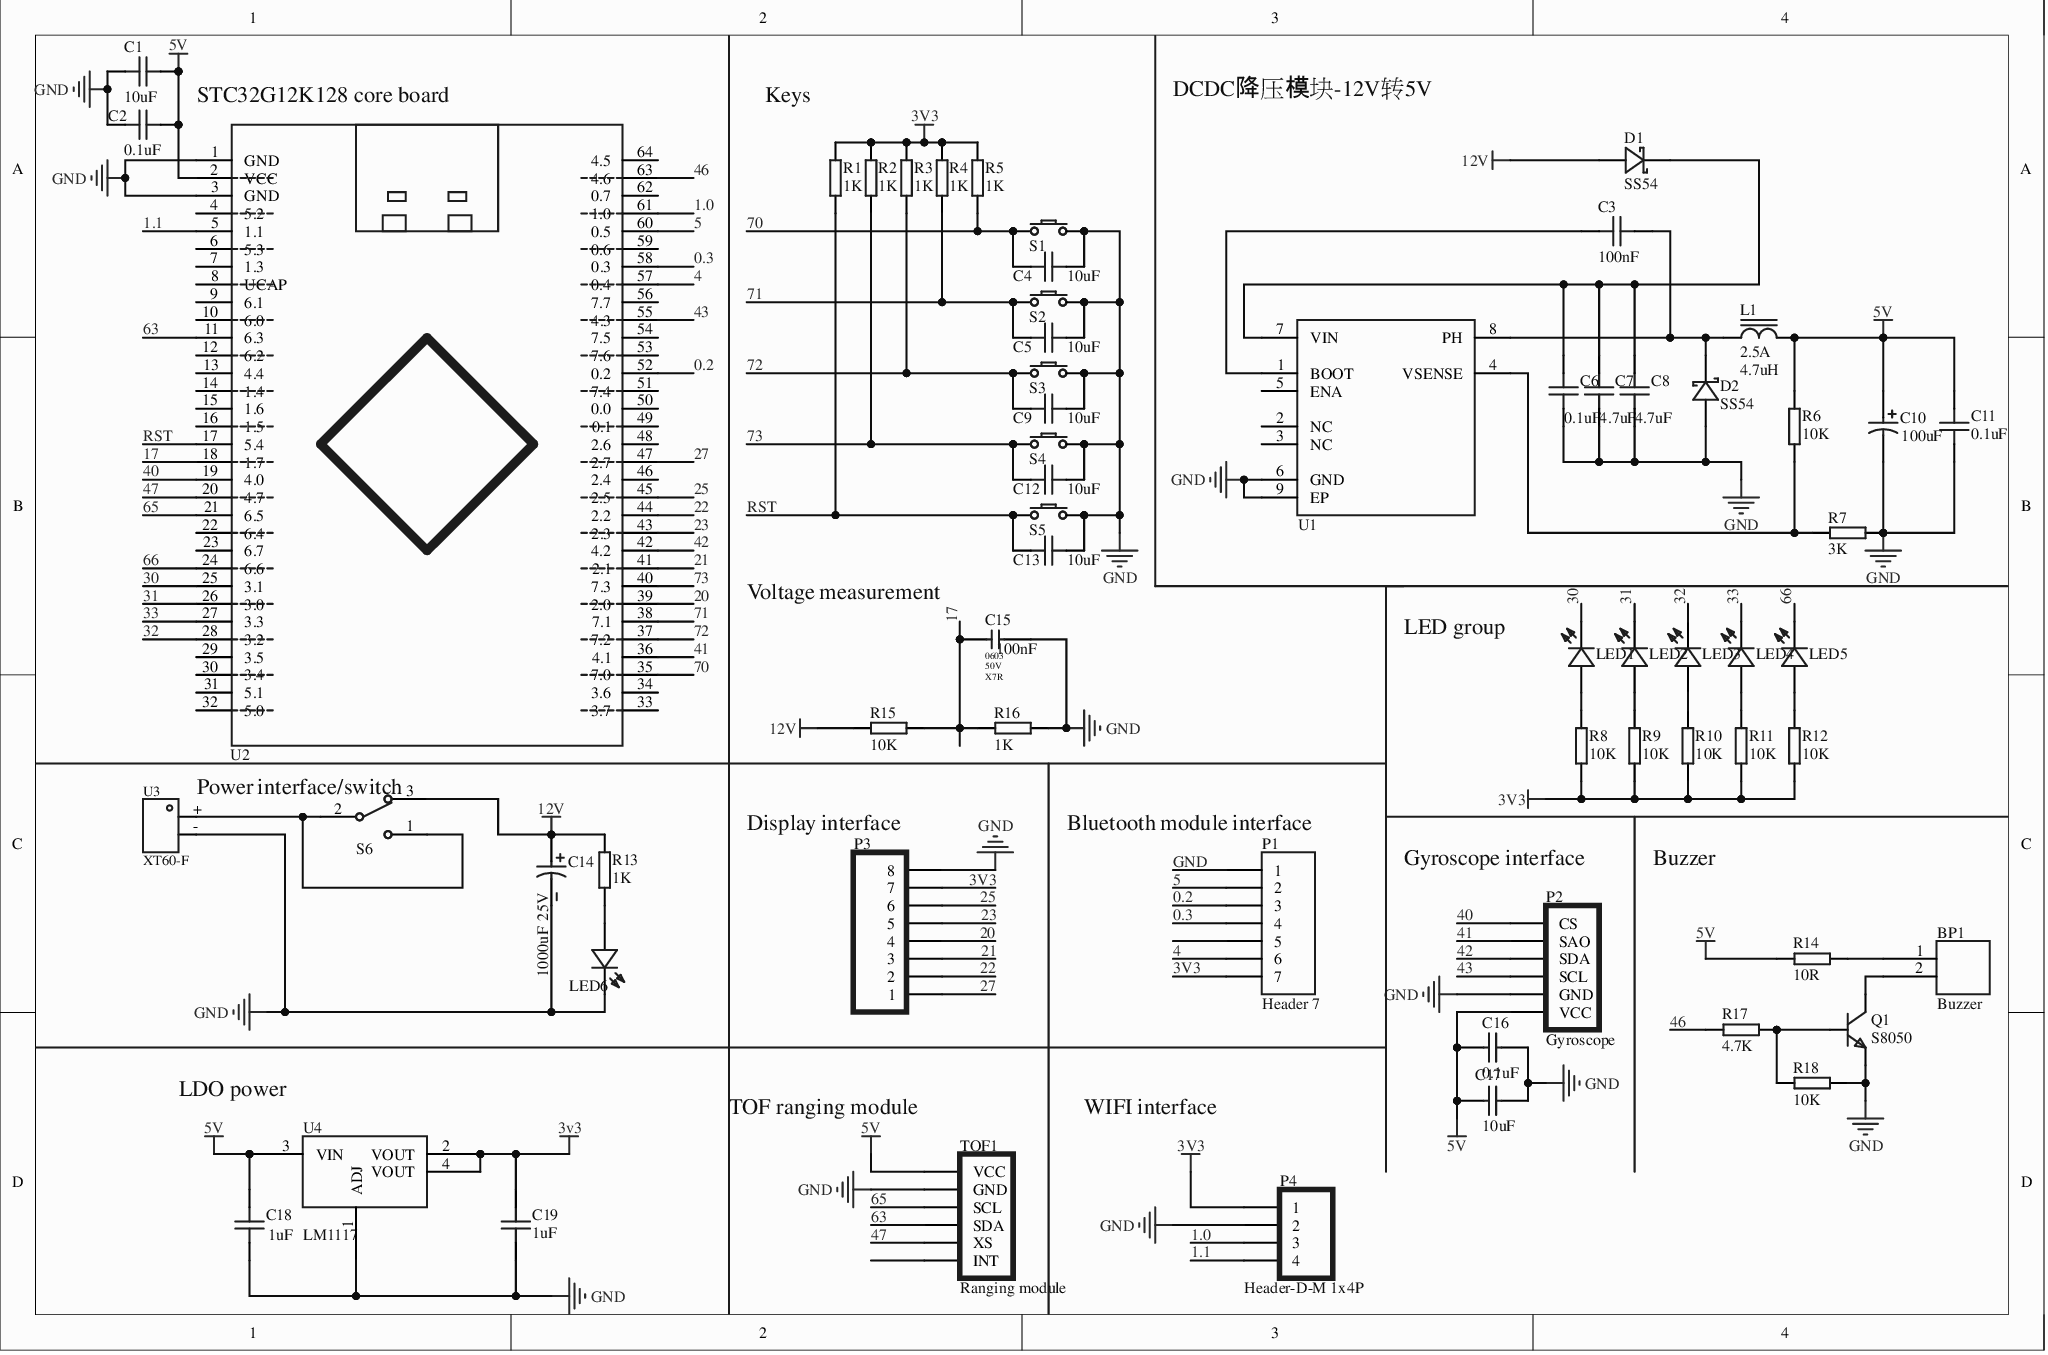
[diagram p0: MISC75116-2.schdoc]
# Altium project MISC75116-3.PrjPcb
1 sheet, 63 parts. Net scope: global (net labels, ports and power ports of the same name join across sheets).
Board file: MISC75116.pcbdoc

## Sheet MISC75116-2.schdoc
size 292 x 193 mm; Name: MISC75116

### Parts
BP1  Buzzer  [5*10fengmiqi]
C1  10uF  [CAPC1608[0603]S-N]
C2  0.1uF  [CAPC1608[0603]S-N]
C3  100nF  [CAPC1608[0603]S-N]
C4  10uF  [CAPC1608[0603]S-N]
C5  10uF  [CAPC1608[0603]S-N]
C6  0.1uF  [CAPC1608[0603]S-N]
C7  4.7uF  [CAPC1608[0603]S-N]
C8  4.7uF  [CAPC1608[0603]S-N]
C9  10uF  [CAPC1608[0603]S-N]
C10  value 100uF  [CAPC1608[0603]S-N]
C11  0.1uF  [CAPC1608[0603]S-N]
C12  10uF  [CAPC1608[0603]S-N]
C13  10uF  [CAPC1608[0603]S-N]
C14  1000uF  25V  [CAPC1608[0603]S-N]
C15  value 100nF  FootPrint: 0603  Voltage: 50V  Type: X7R  [CAPC1608[0603]S-N]
C16  value 0.1uF  [CAPC1608[0603]S-N]
C17  value 10uF  [CAPC1608[0603]S-N]
C18  1uF  [CAPC1608[0603]S-N]
C19  1uF  [CAPC1608[0603]S-N]
D1  SS54  [SOD-123-L]
D2  SS54  [SOD-123-L]
L1  value 4.7uH  Imax: 2.5A  [0402 TPC 4*4*2]
LED1  LED  [LEDC1608(0603)]  (value not drawn)
LED2  LED  [LEDC1608(0603)]  (value not drawn)
LED3  LED  [LEDC1608(0603)]  (value not drawn)
LED4  LED  [LEDC1608(0603)]  (value not drawn)
LED5  LED  [LEDC1608(0603)]  (value not drawn)
LED6  LED  [LEDC1608(0603)]  (value not drawn)
P1  Header 7  [HDR1X7]
P2  Gyroscope  [HDR1X6]
P3  Header  1X8  [HDR1X8]  (value not drawn)
P4  Header-D-M 1x4P  [HDR1X4]
Q1  S8050  [SOT-23]
R1  1K  [RESC1608[0603]S-N]
R2  1K  [RESC1608[0603]S-N]
R3  1K  [RESC1608[0603]S-N]
R4  1K  [RESC1608[0603]S-N]
R5  1K  [RESC1608[0603]S-N]
R6  10K  [RESC1608[0603]S-N]
R7  3K  [RESC1608[0603]S-N]
R8  10K  [RESC1608[0603]S-N]
R9  10K  [RESC1608[0603]S-N]
R10  10K  [RESC1608[0603]S-N]
R11  10K  [RESC1608[0603]S-N]
R12  10K  [RESC1608[0603]S-N]
R13  1K  [RESC1608[0603]S-N]
R14  value 10R  [RESC1608[0603]S-N]
R15  value 10K  [RESC1608[0603]S-N]
R16  value 1K  [RESC1608[0603]S-N]
R17  value 4.7K  [RESC1608[0603]S-N]
R18  value 10K  [RESC1608[0603]S-N]
S1  KEY  [anjiantiepiankaiguan]  (value not drawn)
S2  KEY  [anjiantiepiankaiguan]  (value not drawn)
S3  KEY  [anjiantiepiankaiguan]  (value not drawn)
S4  KEY  [anjiantiepiankaiguan]  (value not drawn)
S5  KEY  [anjiantiepiankaiguan]  (value not drawn)
S6  SW  [SS12D10]  (value not drawn)
TOF1  Ranging module  [HDR1X6]
U1  TPS5450  [5450]  (value not drawn)
U2  STC32G12K128  [STC16F40K128_CoreBoard]  (value not drawn)
U3  XT60-F  [XT60]
U4  LM1117  [LM1117 - duplicate]  (value not drawn)

### Nets
3V3: C19.2 P1.7 P3.7 P4.1 R1.2 R2.2 R3.2 R4.2 R5.2 R8.1 R9.1 R10.1 R11.1 R12.1 U4.2(VOUT) U4.4(VOUT)
5V: C1.2 C2.2 C10.1 C11.2 C16.1 C17.1 C18.2 L1.2 P2.6(VCC) R6.2 R14.1 TOF1.1(VCC) U2.2(VCC) U4.3(VIN)
12V: C14.1 D1.A R13.1 R15.1 S6.3
GND: C1.1 C2.1 C4.2 C5.2 C6.1 C7.1 C8.1 C9.2 C10.2 C11.1 C12.2 C13.2 C14.2 C15.2 C16.2 C17.2 C18.1 C19.1 D2.A LED6.C P1.1 P2.5(GND) P3.8 P4.2 Q1.2(E) R7.2 R16.2 R18.2 S1.1 S2.1 S3.1 S4.1 S5.1 TOF1.2(GND) U1.6(GND) U1.9(EP) U2.1(GND) U2.3(GND) U3.- U4.1(ADJ)
0.2: P1.3 U2.52(0.2)
0.3: P1.4 U2.58(0.3)
1.0: P4.3 U2.61(1.0)
1.1: P4.4 U2.5(1.1)
4: P1.6 U2.57(0.4)
5: P1.2 U2.60(0.5)
17: C15.1 R15.2 R16.1 U2.18(1.7)
20: P3.4 U2.39(2.0)
21: P3.3 U2.41(2.1)
22: P3.2 U2.44(2.2)
23: P3.5 U2.43(2.3)
25: P3.6 U2.45(2.5)
27: P3.1 U2.47(2.7)
30: LED1.C U2.25(3.1)
31: LED2.C U2.26(3.0)
32: LED3.C U2.28(3.2)
33: LED4.C U2.27(3.3)
40: P2.1(CS) U2.19(4.0)
41: P2.2(SAO) U2.36(4.1)
42: P2.3(SDA) U2.42(4.2)
43: P2.4(SCL) U2.55(4.3)
46: R17.1 U2.63(4.6)
47: TOF1.5(XS) U2.20(4.7)
63: TOF1.4(SDA) U2.11(6.3)
65: TOF1.3(SCL) U2.21(6.5)
66: LED5.C U2.24(6.6)
70: C4.1 R5.1 S1.2 U2.35(7.0)
71: C5.1 R4.1 S2.2 U2.38(7.1)
72: C9.1 R3.1 S3.2 U2.37(7.2)
73: C12.1 R2.1 S4.2 U2.40(7.3)
RST: C13.1 R1.1 S5.2 U2.17(5.4)
NetBP1_1: BP1.1 R14.2
NetBP1_2: BP1.2 Q1.3(C)
NetC3_1: C3.1 U1.1(BOOT)
NetC3_2: C3.2 D2.K L1.1 U1.8(PH)
NetC6_2: C6.2 C7.2 C8.2 D1.K U1.7(VIN)
NetLED1_A: LED1.A R8.2
NetLED2_A: LED2.A R9.2
NetLED3_A: LED3.A R10.2
NetLED4_A: LED4.A R11.2
NetLED5_A: LED5.A R12.2
NetLED6_A: LED6.A R13.2
NetQ1_1: Q1.1(B) R17.2 R18.1
NetR6_1: R6.1 R7.1 U1.4(VSENSE)
NetS6_1: S6.1 S6.2 U3.+

Not connected (* = marked no-connect by the designer): P1 5; TOF1 6(INT); U1 2(NC)* 3(NC)* 5(ENA)*; U2 4(5.2) 6(5.3) 7(1.3) 8(UCAP) 9(6.1) 10(6.0) 12(6.2) 13(4.4) 14(1.4) 15(1.6) 16(1.5) 22(6.4) 23(6.7) 29(3.5) 30(3.4) 31(5.1) 32(5.0) 33(3.7) 34(3.6) 46(2.4) 48(2.6) 49(0.1) 50(0.0) 51(7.4) 53(7.6) 54(7.5) 56(7.7) 59(0.6) 62(0.7) 64(4.5)

### Notes on the sheet
- STC32G12K128 core board
- Keys
- DCDC降压模块-12V转5V
- (near C15) Voltage measurement
- LED group
- (near S6) Power interface/switch
- (near P3) Display interface
- (near P1) Bluetooth module interface
- Gyroscope interface
- Buzzer
- (near U4) LDO power
- (near TOF1) TOF ranging module
- WIFI interface
- (near U4) LM1117

### Library data of the parts
BP1 = 蜂鸣器: UniqueId: 13537c3a5c138a7a; SymbolName: Component_1_1; AddInBom: yes; Device: Buzzer; DesignItemID: Component_1_1; LibraryName: STC32G - copy zz; FootprintName: 5*10fengmiqi
C1 = 10uF: SMD capacitor; UniqueId: 5fb4f22ffcb6a001; SymbolName: cap; AddInBom: yes; Device: 10uF; DesignItemID: cap; LibraryName: First-year training board schematic library; FootprintName: CAPC1608[0603]S-N
C2 = 0.1uF: SMD capacitor; UniqueId: 21d50210554cb61f; SymbolName: cap; AddInBom: yes; Device: 0.1uF; DesignItemID: cap; LibraryName: First-year training board schematic library; FootprintName: CAPC1608[0603]S-N
C3 = 100nF: SMD capacitor; UniqueId: ec64484c8c07847f; SymbolName: cap; AddInBom: yes; Device: 100nF; DesignItemID: cap; LibraryName: First-year training board schematic library; FootprintName: CAPC1608[0603]S-N
C4 = 10uF: SMD capacitor; UniqueId: 623e2bb2442f04df; SymbolName: cap; AddInBom: yes; Device: 10uF; DesignItemID: cap; LibraryName: First-year training board schematic library; FootprintName: CAPC1608[0603]S-N
C5 = 10uF: SMD capacitor; UniqueId: 05d417a4d81547fc; SymbolName: cap; AddInBom: yes; Device: 10uF; DesignItemID: cap; LibraryName: First-year training board schematic library; FootprintName: CAPC1608[0603]S-N
C6 = 0.1uF: SMD capacitor; UniqueId: d45ffe04e43665a4; SymbolName: cap; AddInBom: yes; Device: 0.1uF; DesignItemID: cap; LibraryName: First-year training board schematic library; FootprintName: CAPC1608[0603]S-N
C7 = 4.7uF: SMD capacitor; UniqueId: 3007ca2539a35480; SymbolName: cap; AddInBom: yes; Device: 4.7uF; DesignItemID: cap; LibraryName: First-year training board schematic library; FootprintName: CAPC1608[0603]S-N
C8 = 4.7uF: SMD capacitor; UniqueId: 878ab3ab0cce2757; SymbolName: cap; AddInBom: yes; Device: 4.7uF; DesignItemID: cap; LibraryName: First-year training board schematic library; FootprintName: CAPC1608[0603]S-N
C9 = 10uF: SMD capacitor; UniqueId: 60e6893b044e2f17; SymbolName: cap; AddInBom: yes; Device: 10uF; DesignItemID: cap; LibraryName: First-year training board schematic library; FootprintName: CAPC1608[0603]S-N
C10 = =Value+' '+Voltage: Polarized Capacitor (Radial); UniqueId: c1764753ee6525b4; SymbolName: Cap-Elect; AddInBom: yes; Device: 100uF; Published: 8-Jun-2000; Revision: July-2002: Re-released for DXP Platform.; Price(RMB): 0.000; DesignItemID: Cap-Elect; LibraryName: STC32G - copy zz; FootprintName: CAPC1608[0603]S-N; Publisher: COMPANY_A
C11 = 0.1uF: SMD capacitor; UniqueId: b49c3108c5288e9f; SymbolName: cap; AddInBom: yes; Device: 0.1uF; DesignItemID: cap; LibraryName: First-year training board schematic library; FootprintName: CAPC1608[0603]S-N
C12 = 10uF: SMD capacitor; UniqueId: 4eba2014d94c20ef; SymbolName: cap; AddInBom: yes; Device: 10uF; DesignItemID: cap; LibraryName: First-year training board schematic library; FootprintName: CAPC1608[0603]S-N
C13 = 10uF: SMD capacitor; UniqueId: 8d11a04c32f33369; SymbolName: cap; AddInBom: yes; Device: 10uF; DesignItemID: cap; LibraryName: First-year training board schematic library; FootprintName: CAPC1608[0603]S-N
C14 = 1000uF  25V: Through-hole electrolytic capacitor; UniqueId: c9f451b8b2c5f180; SymbolName: cap_ZhiCha; AddInBom: yes; Device: 1000uF  25V; DesignItemID: cap_ZhiCha; LibraryName: First-year training board schematic library; FootprintName: CAPC1608[0603]S-N
C15 = =Value +' '+ Voltage + ' ' + Type: SMD ceramic capacitor; MLCC; 0603(1608);; Device: 100nF 50V X7R; UniqueId: 4a0fa0f8d5a09ecc; SymbolName: 100nF 0603 50V X7R; AddInBom: yes; Revision: V1.0; DesignItemID: 100nF 0603 50V X7R; LibraryName: STC8H&16F&32G_board_V3.0; FootprintName: CAPC1608[0603]S-N
C16 = =Value + ' ' + Tolerance +' '+ Voltage: SMD capacitor; Device: 0.1uF ±10% 25V; Voltage: 25V; Tolerance: ±10%; UniqueId: 6992a3033003bbbd; SymbolName: Cap-Chip_4; AddInBom: yes; Published: 8-Jun-2000; Revision: July-2002: Re-released for DXP Platform.; Price(RMB): 0.000; Origin Footprint: CAPC1608[0603]S-N; OriginFootprint 2: CAPC1608[0603]S-N; DesignItemID: Cap-Chip_4; LibraryName: STC32G - copy zz; FootprintName: CAPC1608[0603]S-N; Publisher: COMPANY_A
C17 = =Value + ' ' + Tolerance +' '+ Voltage_1: SMD capacitor; Voltage: 50V; Tolerance: ±10%; UniqueId: 5e7964c847a08933; SymbolName: Cap-Chip_2; AddInBom: yes; Device: =Value + ' ' + Tolerance +' '+ Voltage_1; Published: 8-Jun-2000; Revision: July-2002: Re-released for DXP Platform.; Price(RMB): 0.000; Origin Footprint: CAPC1608[0603]S-N; DesignItemID: Cap-Chip_2; LibraryName: STC32G - copy zz; FootprintName: CAPC1608[0603]S-N; Publisher: COMPANY_A
C18 = 1uF: SMD capacitor; UniqueId: 9b976857f3e39318; SymbolName: cap; AddInBom: yes; Device: 1uF; DesignItemID: cap; LibraryName: First-year training board schematic library; FootprintName: CAPC1608[0603]S-N
C19 = 1uF: SMD capacitor; UniqueId: 7dc0401965f49c44; SymbolName: cap; AddInBom: yes; Device: 1uF; DesignItemID: cap; LibraryName: First-year training board schematic library; FootprintName: CAPC1608[0603]S-N
D1 = SS54: SS54 Schottky diode; UniqueId: 07a0d5848cd81316; AddInBom: yes; OriginModelName: SOD-123; Device: SS54; Revision: V1.0; Value: SS54; DesignItemID: SS54; LibraryName: STC32F_48P_CCD_board_V1.1; SymbolName: SS54; FootprintName: SOD-123-L
D2 = SS54: SS54 Schottky diode; UniqueId: fa5cd661465da5bc; AddInBom: yes; OriginModelName: SOD-123; Device: SS54; Revision: V1.0; Value: SS54; DesignItemID: SS54; LibraryName: STC32F_48P_CCD_board_V1.1; SymbolName: SS54; FootprintName: SOD-123-L
L1 = =Value + ' ' + Imax: Power inductor; Device: 4.7uH 2.5A; DCR: .5m; UniqueId: 2f42939b1ffc8518; SymbolName: Ind-Power; AddInBom: yes; Published: 8-Jun-2000; Revision: July-2002: Re-released for DXP Platform.; Price(RMB): 0.000; DesignItemID: Ind-Power; LibraryName: STC32G - copy zz; FootprintName: 0402 TPC 4*4*2; Publisher: COMPANY_A
LED1 = LED: SMD LED; UniqueId: a4c4b307afb8d999; AddInBom: yes; OriginModelName: 0603 (1608) LED Base (Separate Lens); Device: LED; DesignItemID: LED; LibraryName: First-year training board schematic library; SymbolName: LED; FootprintName: LEDC1608(0603)
LED2 = LED: SMD LED; UniqueId: a245eb2d2aad9559; AddInBom: yes; OriginModelName: 0603 (1608) LED Base (Separate Lens); Device: LED; DesignItemID: LED; LibraryName: First-year training board schematic library; SymbolName: LED; FootprintName: LEDC1608(0603)
LED3 = LED: SMD LED; UniqueId: 01e448f2d6732d04; AddInBom: yes; OriginModelName: 0603 (1608) LED Base (Separate Lens); Device: LED; DesignItemID: LED; LibraryName: First-year training board schematic library; SymbolName: LED; FootprintName: LEDC1608(0603)
LED4 = LED: SMD LED; UniqueId: c2d123990b1fde2c; AddInBom: yes; OriginModelName: 0603 (1608) LED Base (Separate Lens); Device: LED; DesignItemID: LED; LibraryName: First-year training board schematic library; SymbolName: LED; FootprintName: LEDC1608(0603)
LED5 = LED: SMD LED; UniqueId: 1218a8b603bcfedf; AddInBom: yes; OriginModelName: 0603 (1608) LED Base (Separate Lens); Device: LED; DesignItemID: LED; LibraryName: First-year training board schematic library; SymbolName: LED; FootprintName: LEDC1608(0603)
LED6 = LED: SMD LED; UniqueId: 1801f051ed571ab9; AddInBom: yes; OriginModelName: 0603 (1608) LED Base (Separate Lens); Device: LED; DesignItemID: LED; LibraryName: First-year training board schematic library; SymbolName: LED; FootprintName: LEDC1608(0603)
P1 = Header 7: Header, 7-Pin; UniqueId: f88e3064cb77b82c; AddInBom: yes; Device: Header 7; LatestRevisionDate: 17-Jul-2002; LatestRevisionNote: Re-released for DXP Platform.; DesignItemID: Header 7; LibraryName: STC32G - copy zz; SymbolName: Header 7; FootprintName: HDR1X7; Publisher: COMPANY_A
P2 = 陀螺仪: Header, 6-Pin; UniqueId: ddb6c992c6045fb8; SymbolName: Header 6; AddInBom: yes; Device: Gyroscope; LatestRevisionDate: 17-Jul-2002; LatestRevisionNote: Re-released for DXP Platform.; Price(RMB): 0.00; DesignItemID: Header 6; LibraryName: STC32G - copy zz; FootprintName: HDR1X6; Publisher: COMPANY_A
P3 = Header  1X8: 1X8; UniqueId: 10472a1c2ba3b044; AddInBom: yes; OriginModelName: 1001-8; Device: Header  1X8; DesignItemID: Header  1X8; LibraryName: First-year training board schematic library; SymbolName: Header  1X8; FootprintName: HDR1X8
P4 = Header-D-M 1x4P: 1x4pin, through-hole, pin header; UniqueId: 28b6bd94bccb65c1; AddInBom: yes; Device: Header-D-M 1x4P; Revision: V1.0; Value: Header-D-M 1x4P; DesignItemID: Header-D-M 1x4P; LibraryName: STC32G - copy zz; SymbolName: Header-D-M 1x4P; FootprintName: HDR1X4
Q1 = S8050: Discrete NPN Bipolar Transistor; UniqueId: 047b734180970fea; SymbolName: NPN S8050; AddInBom: yes; OriginModelName: SOT-23-3P; ModelTransform: v2:[-7.232166136696968e-15,-39.37007874015748,0,39.37007874015748,-7.232166136696968e-15,0,0,0,39.37007874015748,0.0024,-0.0032,0]; ModelId: dd91bed6c7114a8387ef499cf979050b; Device: S8050; Published: 8-Jun-2000; Revision: July-2002: Re-released for DXP Platform.; Price(RMB): 0.000; PartNumber: S8050; DesignItemID: NPN S8050; LibraryName: STC32G - copy zz; FootprintName: SOT-23; ModelName: SOT-23; Publisher: COMPANY_A
R1 = 1K: SMD resistor; UniqueId: 4e166b190d4de1c3; SymbolName: RES; AddInBom: yes; OriginModelName: R0603; ModelTransform: v2:[39.37007874015748,0,0,0,39.37007874015748,0,0,0,39.37007874015748,0.0032,0.0034,0]; ModelId: fc143cca1e79419f9cd78b61e9279f08; Device: 1K; DesignItemID: RES; LibraryName: First-year training board schematic library; FootprintName: RESC1608[0603]S-N; ModelName: R0603
R2 = 1K: SMD resistor; UniqueId: 06442d24ab060343; SymbolName: RES; AddInBom: yes; OriginModelName: R0603; ModelTransform: v2:[39.37007874015748,0,0,0,39.37007874015748,0,0,0,39.37007874015748,0.0032,0.0034,0]; ModelId: fc143cca1e79419f9cd78b61e9279f08; Device: 1K; DesignItemID: RES; LibraryName: First-year training board schematic library; FootprintName: RESC1608[0603]S-N; ModelName: R0603
R3 = 1K: SMD resistor; UniqueId: 6e26aea592918673; SymbolName: RES; AddInBom: yes; OriginModelName: R0603; ModelTransform: v2:[39.37007874015748,0,0,0,39.37007874015748,0,0,0,39.37007874015748,0.0032,0.0034,0]; ModelId: fc143cca1e79419f9cd78b61e9279f08; Device: 1K; DesignItemID: RES; LibraryName: First-year training board schematic library; FootprintName: RESC1608[0603]S-N; ModelName: R0603
R4 = 1K: SMD resistor; UniqueId: 49359f7360e76581; SymbolName: RES; AddInBom: yes; OriginModelName: R0603; ModelTransform: v2:[39.37007874015748,0,0,0,39.37007874015748,0,0,0,39.37007874015748,0.0032,0.0034,0]; ModelId: fc143cca1e79419f9cd78b61e9279f08; Device: 1K; DesignItemID: RES; LibraryName: First-year training board schematic library; FootprintName: RESC1608[0603]S-N; ModelName: R0603
R5 = 1K: SMD resistor; UniqueId: 96bd3269827a783e; SymbolName: RES; AddInBom: yes; OriginModelName: R0603; ModelTransform: v2:[39.37007874015748,0,0,0,39.37007874015748,0,0,0,39.37007874015748,0.0032,0.0034,0]; ModelId: fc143cca1e79419f9cd78b61e9279f08; Device: 1K; DesignItemID: RES; LibraryName: First-year training board schematic library; FootprintName: RESC1608[0603]S-N; ModelName: R0603
R6 = 10K: SMD resistor; UniqueId: c9a24d22ca7022dc; SymbolName: RES; AddInBom: yes; OriginModelName: R0603; ModelTransform: v2:[39.37007874015748,0,0,0,39.37007874015748,0,0,0,39.37007874015748,0.0032,0.0034,0]; ModelId: fc143cca1e79419f9cd78b61e9279f08; Device: 10K; DesignItemID: RES; LibraryName: First-year training board schematic library; FootprintName: RESC1608[0603]S-N; ModelName: R0603
R7 = 3K: SMD resistor; UniqueId: 01f5c70ff2630ee7; SymbolName: RES; AddInBom: yes; OriginModelName: R0603; ModelTransform: v2:[39.37007874015748,0,0,0,39.37007874015748,0,0,0,39.37007874015748,0.0032,0.0034,0]; ModelId: fc143cca1e79419f9cd78b61e9279f08; Device: 3K; DesignItemID: RES; LibraryName: First-year training board schematic library; FootprintName: RESC1608[0603]S-N; ModelName: R0603
R8 = 10K: SMD resistor; UniqueId: f0665cc51e401020; SymbolName: RES; AddInBom: yes; OriginModelName: R0603; ModelTransform: v2:[39.37007874015748,0,0,0,39.37007874015748,0,0,0,39.37007874015748,0.0032,0.0034,0]; ModelId: fc143cca1e79419f9cd78b61e9279f08; Device: 10K; DesignItemID: RES; LibraryName: First-year training board schematic library; FootprintName: RESC1608[0603]S-N; ModelName: R0603
R9 = 10K: SMD resistor; UniqueId: 7a9d276dcc23a651; SymbolName: RES; AddInBom: yes; OriginModelName: R0603; ModelTransform: v2:[39.37007874015748,0,0,0,39.37007874015748,0,0,0,39.37007874015748,0.0032,0.0034,0]; ModelId: fc143cca1e79419f9cd78b61e9279f08; Device: 10K; DesignItemID: RES; LibraryName: First-year training board schematic library; FootprintName: RESC1608[0603]S-N; ModelName: R0603
R10 = 10K: SMD resistor; UniqueId: 7663007c1f2bc029; SymbolName: RES; AddInBom: yes; OriginModelName: R0603; ModelTransform: v2:[39.37007874015748,0,0,0,39.37007874015748,0,0,0,39.37007874015748,0.0032,0.0034,0]; ModelId: fc143cca1e79419f9cd78b61e9279f08; Device: 10K; DesignItemID: RES; LibraryName: First-year training board schematic library; FootprintName: RESC1608[0603]S-N; ModelName: R0603
R11 = 10K: SMD resistor; UniqueId: 069ba0dc55a84bc8; SymbolName: RES; AddInBom: yes; OriginModelName: R0603; ModelTransform: v2:[39.37007874015748,0,0,0,39.37007874015748,0,0,0,39.37007874015748,0.0032,0.0034,0]; ModelId: fc143cca1e79419f9cd78b61e9279f08; Device: 10K; DesignItemID: RES; LibraryName: First-year training board schematic library; FootprintName: RESC1608[0603]S-N; ModelName: R0603
R12 = 10K: SMD resistor; UniqueId: f574a6082c36e6cb; SymbolName: RES; AddInBom: yes; OriginModelName: R0603; ModelTransform: v2:[39.37007874015748,0,0,0,39.37007874015748,0,0,0,39.37007874015748,0.0032,0.0034,0]; ModelId: fc143cca1e79419f9cd78b61e9279f08; Device: 10K; DesignItemID: RES; LibraryName: First-year training board schematic library; FootprintName: RESC1608[0603]S-N; ModelName: R0603
R13 = 1K: SMD resistor; UniqueId: ff7631ddbc1e2fda; SymbolName: RES; AddInBom: yes; OriginModelName: R0603; ModelTransform: v2:[39.37007874015748,0,0,0,39.37007874015748,0,0,0,39.37007874015748,0.0032,0.0034,0]; ModelId: fc143cca1e79419f9cd78b61e9279f08; Device: 1K; DesignItemID: RES; LibraryName: First-year training board schematic library; FootprintName: RESC1608[0603]S-N; ModelName: R0603
R14 = =Value+' '+Tolerance_2: SMD resistor; Tolerance: ±1%; UniqueId: d58291ee940aacae; SymbolName: Res-Chip_6; AddInBom: yes; OriginModelName: R0603; ModelTransform: v2:[39.37007874015748,0,0,0,39.37007874015748,0,0,0,39.37007874015748,0.0032,0.0034,0]; ModelId: fc143cca1e79419f9cd78b61e9279f08; Device: =Value+' '+Tolerance_2; Published: 8-Jun-2000; Revision: July-2002: Re-released for DXP Platform.; Price(RMB): 0.000; DesignItemID: Res-Chip_6; LibraryName: STC32G - copy zz; FootprintName: RESC1608[0603]S-N; ModelName: R0603; Publisher: COMPANY_A
R15 = =Value+' '+Tolerance_1: SMD resistor; Power: 1/8W; Tolerance: ±1%; UniqueId: 615753eb74f5e235; SymbolName: Res-Chip_2; AddInBom: yes; OriginModelName: R0603; ModelTransform: v2:[39.37007874015748,0,0,0,39.37007874015748,0,0,0,39.37007874015748,0.0032,0.0034,0]; ModelId: fc143cca1e79419f9cd78b61e9279f08; Device: =Value+' '+Tolerance_1; Revision: V1.0; DesignItemID: Res-Chip_2; LibraryName: STC8H&16F&32G_board_V3.0; FootprintName: RESC1608[0603]S-N; ModelName: R0603
R16 = =Value+' '+Tolerance: SMD resistor; Device: 1K ±1%; Power: 1/8W; Tolerance: ±1%; UniqueId: 49a4252fe0d0166e; SymbolName: Res-Chip_3; AddInBom: yes; OriginModelName: R0603; ModelTransform: v2:[39.37007874015748,0,0,0,39.37007874015748,0,0,0,39.37007874015748,0.0032,0.0034,0]; ModelId: fc143cca1e79419f9cd78b61e9279f08; Revision: V1.0; DesignItemID: Res-Chip_3; LibraryName: STC8H&16F&32G_board_V3.0; FootprintName: RESC1608[0603]S-N; ModelName: R0603
R17 = =Value+' '+Tolerance_3: SMD resistor; Tolerance: ±1%; UniqueId: 7917acf7ef76b3a3; SymbolName: Res-Chip; AddInBom: yes; OriginModelName: R0603; ModelTransform: v2:[39.37007874015748,0,0,0,39.37007874015748,0,0,0,39.37007874015748,0.0032,0.0034,0]; ModelId: fc143cca1e79419f9cd78b61e9279f08; Device: =Value+' '+Tolerance_3; Published: 8-Jun-2000; Revision: July-2002: Re-released for DXP Platform.; Price(RMB): 0.000; DesignItemID: Res-Chip; LibraryName: STC32G - copy zz; FootprintName: RESC1608[0603]S-N; ModelName: R0603; Publisher: COMPANY_A
R18 = =Value+' '+Tolerance: SMD resistor; Device: 10K ±1%; Tolerance: ±1%; UniqueId: 1bd7cdeea74e381f; SymbolName: Res-Chip_3; Power: 1/8W; AddInBom: yes; OriginModelName: R0603; ModelTransform: v2:[39.37007874015748,0,0,0,39.37007874015748,0,0,0,39.37007874015748,0.0032,0.0034,0]; ModelId: fc143cca1e79419f9cd78b61e9279f08; Published: 8-Jun-2000; Revision: July-2002: Re-released for DXP Platform.; Price(RMB): 0.000; DesignItemID: Res-Chip_3; LibraryName: STC32G - copy zz; FootprintName: RESC1608[0603]S-N; ModelName: R0603; Publisher: COMPANY_A
S1 = KEY: Keys; UniqueId: da892dff24010eb4; AddInBom: yes; Device: KEY; DesignItemID: KEY; LibraryName: First-year training board schematic library; SymbolName: KEY; FootprintName: anjiantiepiankaiguan
S2 = KEY: Keys; UniqueId: b3b756e6393b620b; AddInBom: yes; Device: KEY; DesignItemID: KEY; LibraryName: First-year training board schematic library; SymbolName: KEY; FootprintName: anjiantiepiankaiguan
S3 = KEY: Keys; UniqueId: 7b79a888bb89fb64; AddInBom: yes; Device: KEY; DesignItemID: KEY; LibraryName: First-year training board schematic library; SymbolName: KEY; FootprintName: anjiantiepiankaiguan
S4 = KEY: Keys; UniqueId: 5bcf7e05ad3bc526; AddInBom: yes; Device: KEY; DesignItemID: KEY; LibraryName: First-year training board schematic library; SymbolName: KEY; FootprintName: anjiantiepiankaiguan
S5 = KEY: Keys; UniqueId: 3819b3f665fa52ad; AddInBom: yes; Device: KEY; DesignItemID: KEY; LibraryName: First-year training board schematic library; SymbolName: KEY; FootprintName: anjiantiepiankaiguan
S6 = SW: SPDT switch; UniqueId: 9387c3ba9aa20518; AddInBom: yes; OriginModelName: ms-13aap1; Device: SW; DesignItemID: SW; LibraryName: First-year training board schematic library; SymbolName: SW; FootprintName: SS12D10
TOF1 = 测距模块: Header, 6-Pin; UniqueId: de50b61311c4a74b; SymbolName: Header 6_1; AddInBom: yes; OriginModelName: 1001-6; Device: Ranging module; LatestRevisionDate: 17-Jul-2002; LatestRevisionNote: Re-released for DXP Platform.; Price(RMB): 0.00; DesignItemID: Header 6_1; LibraryName: STC32G - copy zz; FootprintName: HDR1X6; Publisher: COMPANY_A
U1 = TPS5450: 5v regulator chip; UniqueId: 48a4a086d8c42a18; AddInBom: yes; Device: TPS5450; DesignItemID: TPS5450; LibraryName: First-year training board schematic library; SymbolName: TPS5450; FootprintName: 5450
U2 = STC32G12K128: STC32G12K128 core board; UniqueId: d74c11912b695046; AddInBom: yes; Device: STC32G12K128; DesignItemID: STC32G12K128; LibraryName: First-year training board schematic library; SymbolName: STC32G12K128; FootprintName: STC16F40K128_CoreBoard
U3 = XT60-F: UniqueId: eac3f191c372887e; AddInBom: yes; Device: XT60-F; DesignItemID: XT60-F; LibraryName: STC32G - copy zz; SymbolName: XT60-F; FootprintName: XT60
U4 = LM1117: 3.3V regulator; UniqueId: e5d1bee62801ccc5; AddInBom: yes; Device: LM1117; DesignItemID: LM1117; LibraryName: First-year training board schematic library; SymbolName: LM1117; FootprintName: LM1117 - duplicate